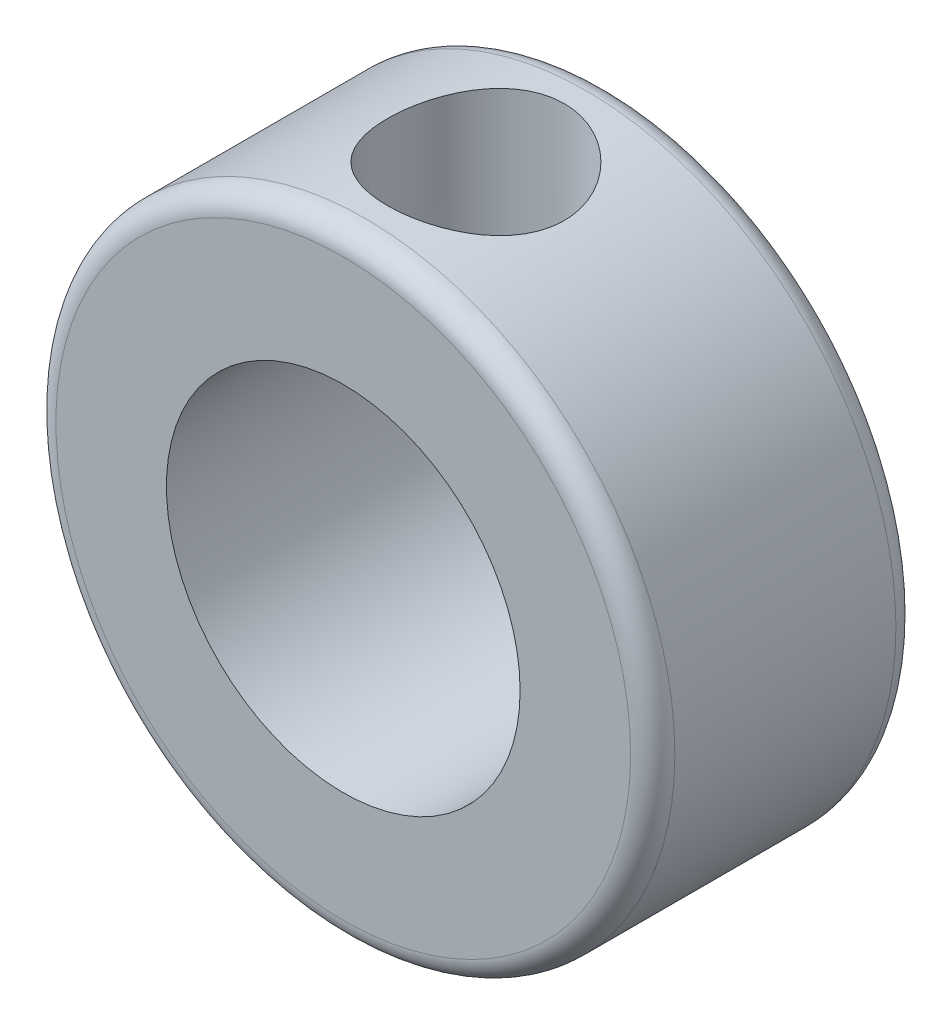
SolidWorks part; units mm, degrees
ref_plane "Front Plane" through (0, 0, 0) normal (0, 0, 1) x (1, 0, 0)
ref_plane "Top Plane" through (0, 0, 0) normal (0, 1, 0) x (1, 0, 0)
ref_plane "Right Plane" through (0, 0, 0) normal (1, 0, 0) x (0, 0, -1)
sketch "Sketch1" plane through (0, 0, 0) normal (0, 0, 1) x (1, 0, 0)
  circle A0 centre (0, 0) radius 8
  circle A1 centre (0, 0) radius 14
  dimension "D1" = 16
  dimension "D2" = 28
extrude "Boss-Extrude1" add sketch "Sketch1" along normal mid plane 12
fillet "Fillet1" radius 1 2 edges at (14, 0, -6) (14, 0, 6)
sketch "Sketch2" plane through (0, 0, 0) normal (0, 1, 0) x (1, 0, 0)
  circle A0 centre (0, 0) radius 4
  dimension "D1" = 8
extrude "Cut-Extrude1" cut sketch "Sketch2" along normal blind 20
